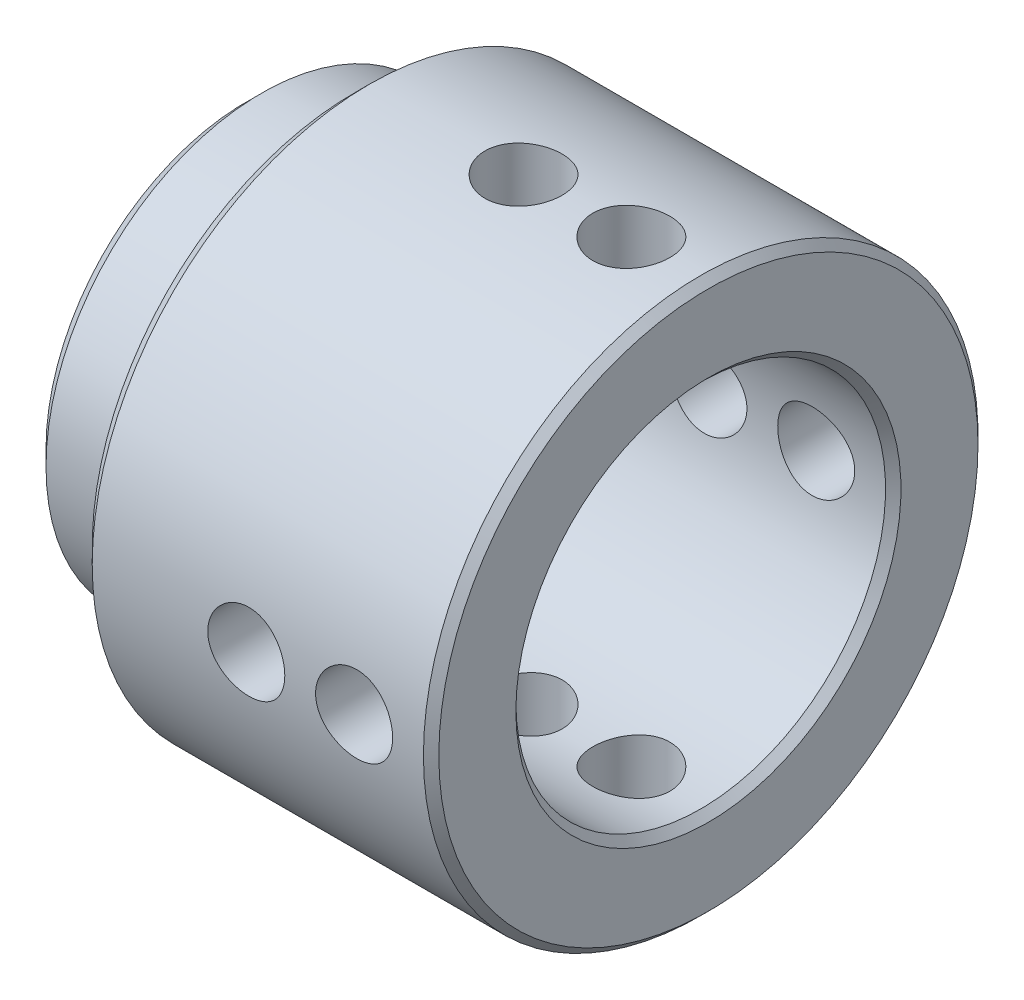
from build123d import *

# Parameters (mm, degrees)
SKETCH_2_W               = 4
SKETCH_2_H               = 6.5
CUT_EXTRUDE_1_DEPTH      = 40.344631146
CUT_EXTRUDE_2_DEPTH      = 40.344631146
CUT_EXTRUDE_2_DEPTH_BACK = 40.344631146
SKETCH_3_R               = 2.5
CHAMFER_1_SIZE           = 1
CHAMFER_2_SIZE           = 0.5
CUT_EXTRUDE_3_DEPTH      = 40.344631238
CUT_EXTRUDE_3_DEPTH_BACK = 40.344631238
SKETCH_4_R               = 2.5


with BuildPart() as part:
    # 草图1 → 旋转1 (revolve)
    with BuildSketch(Plane.XY, mode=Mode.PRIVATE) as revolve_1_sk:
        Polygon((0, 5), (12, 5), (12, 12), (30, 12), (30, 18), (7, 18), (7, 14), (0, 14), align=None)
    revolve(revolve_1_sk.sketch.rotate(Axis((0, 0, 0), (1, 0, 0)), 90), axis=Axis((0, 0, 0), (1, 0, 0)))

    # 草图2 → 切除-拉伸1 (cut, through all)
    with BuildSketch(Plane.ZY):
        with Locations((0, 3.25)):
            Rectangle(SKETCH_2_W, SKETCH_2_H)
    extrude(amount=-CUT_EXTRUDE_1_DEPTH, mode=Mode.SUBTRACT)

    # 草图3 → 切除-拉伸2 (cut, two sides: drawn at the far end of the back side and taken through both)
    with BuildSketch(Plane(origin=(0, 0, 0), x_dir=(1, 0, 0), z_dir=(0, 1, 0)).offset(-CUT_EXTRUDE_2_DEPTH_BACK)):
        with Locations(Location((18, 0, 0), (0, 0, 270))):
            Circle(SKETCH_3_R)
        with Locations(Location((25, 0, 0), (0, 0, 270))):
            Circle(SKETCH_3_R)
    extrude(amount=CUT_EXTRUDE_2_DEPTH + CUT_EXTRUDE_2_DEPTH_BACK, mode=Mode.SUBTRACT)

    # 倒角1
    chamfer_1_edges = [part.edges().sort_by_distance(p)[0] for p in [
        (0, 0, -14),
        (7, 0, -18),
    ]]
    chamfer(chamfer_1_edges, length=CHAMFER_1_SIZE)

    # 倒角2
    chamfer_2_edges = [part.edges().sort_by_distance(p)[0] for p in [
        (30, 0, -18),
        (30, 0, -12),
    ]]
    chamfer(chamfer_2_edges, length=CHAMFER_2_SIZE)

    # 草图4 → 切除-拉伸3 (cut, two sides: drawn at the far end of the back side and taken through both)
    with BuildSketch(Plane.XY.offset(-CUT_EXTRUDE_3_DEPTH_BACK)):
        with Locations((25, 0)):
            Circle(SKETCH_4_R)
        with Locations((18, 0)):
            Circle(SKETCH_4_R)
    extrude(amount=CUT_EXTRUDE_3_DEPTH + CUT_EXTRUDE_3_DEPTH_BACK, mode=Mode.SUBTRACT)


solid = part.part
